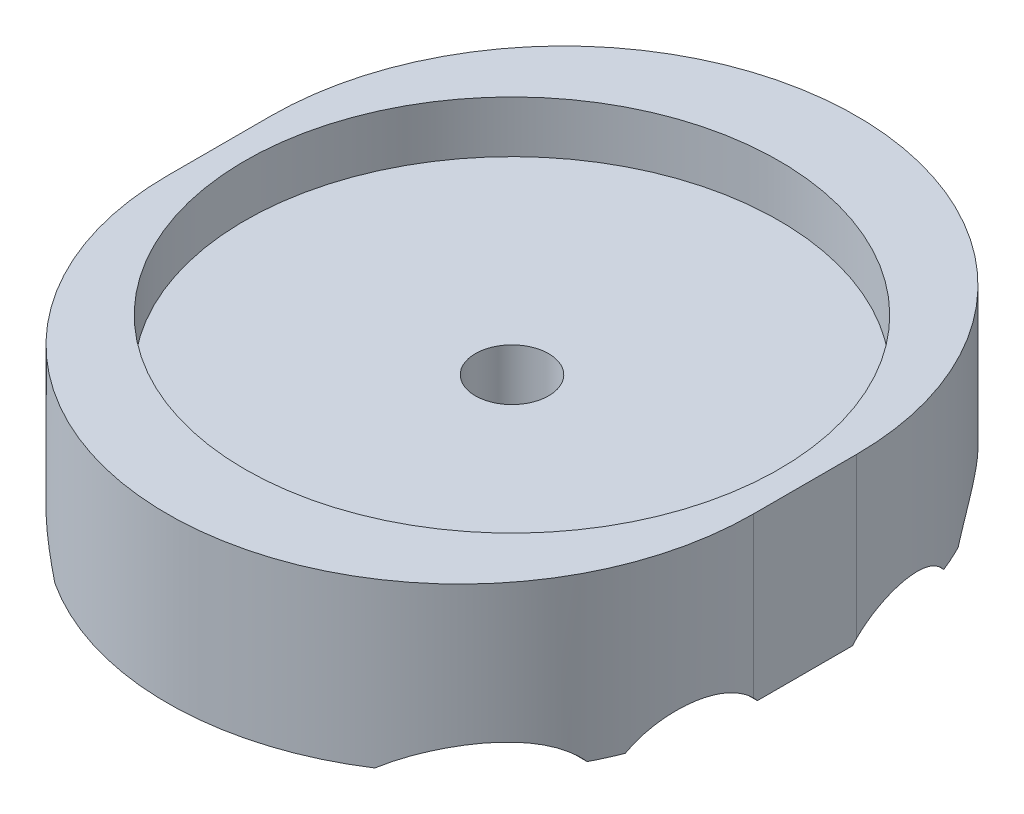
from build123d import *

# Parameters (mm, degrees)
EXTRUDE_1_DEPTH          = 19
SKETCH_2_R               = 31
CUT_EXTRUDE_1_DEPTH      = 6
HOLE_WIZARD_M10_1_D      = 8.5
HOLE_WIZARD_M10_1_DEPTH  = 6
HOLE_WIZARD_M10_1_TIP    = 2.553657631
CUT_EXTRUDE_2_DEPTH      = 56.830099409
CUT_EXTRUDE_2_DEPTH_BACK = 56.830099409
SKETCH_5_R               = 8.5


with BuildPart() as part:
    # 草图1 → 凸台-拉伸1 (new body)
    with BuildSketch(Plane(origin=(0, 0, 0), x_dir=(1, 0, 0), z_dir=(0, 1, 0))):
        with BuildLine():
            Line((34, -6), (34, 6))
            ThreePointArc((34, 6), (0, 40), (-34, 6))
            Line((-34, 6), (-34, -6))
            ThreePointArc((-34, -6), (0, -40), (34, -6))
        make_face()
    extrude(amount=EXTRUDE_1_DEPTH)

    # 草图2 → 切除-拉伸1 (cut)
    with BuildSketch(Plane(origin=(0, 19, 0), x_dir=(1, 0, 0), z_dir=(0, 1, 0))):
        with Locations(Location((0, 0, 0), (0, 0, 270))):
            Circle(SKETCH_2_R)
    extrude(amount=-CUT_EXTRUDE_1_DEPTH, mode=Mode.SUBTRACT)

    # M10 螺纹孔1
    with Locations(Plane(origin=(0, 13, 0), x_dir=(1, 0, 0), z_dir=(0, 1, 0))):
        with Locations((0, 0)):
            Hole(HOLE_WIZARD_M10_1_D / 2, depth=HOLE_WIZARD_M10_1_DEPTH)
            with Locations((0, 0, -(HOLE_WIZARD_M10_1_DEPTH + HOLE_WIZARD_M10_1_TIP / 2))):  # 118° drill point
                Cone(0, HOLE_WIZARD_M10_1_D / 2, HOLE_WIZARD_M10_1_TIP, mode=Mode.SUBTRACT)

    # 草图5 → 切除-拉伸2 (cut, two sides: drawn at the far end of the back side and taken through both)
    with BuildSketch(Plane(origin=(0, 0, 0), x_dir=(0, 0, -1), z_dir=(1, 0, 0)).offset(-CUT_EXTRUDE_2_DEPTH_BACK)):
        with Locations((28, -5.5)):
            Circle(SKETCH_5_R)
        with Locations((12, -5.5)):
            Circle(SKETCH_5_R)
        with Locations((12, -5.5)):
            Circle(SKETCH_5_R)
        with Locations((28, -5.5)):
            Circle(SKETCH_5_R)
        with Locations((-28, -5.5)):
            Circle(SKETCH_5_R)
        with Locations((-12, -5.5)):
            Circle(SKETCH_5_R)
        with Locations((-12, -5.5)):
            Circle(SKETCH_5_R)
        with Locations((-28, -5.5)):
            Circle(SKETCH_5_R)
    extrude(amount=CUT_EXTRUDE_2_DEPTH + CUT_EXTRUDE_2_DEPTH_BACK, mode=Mode.SUBTRACT)


solid = part.part
